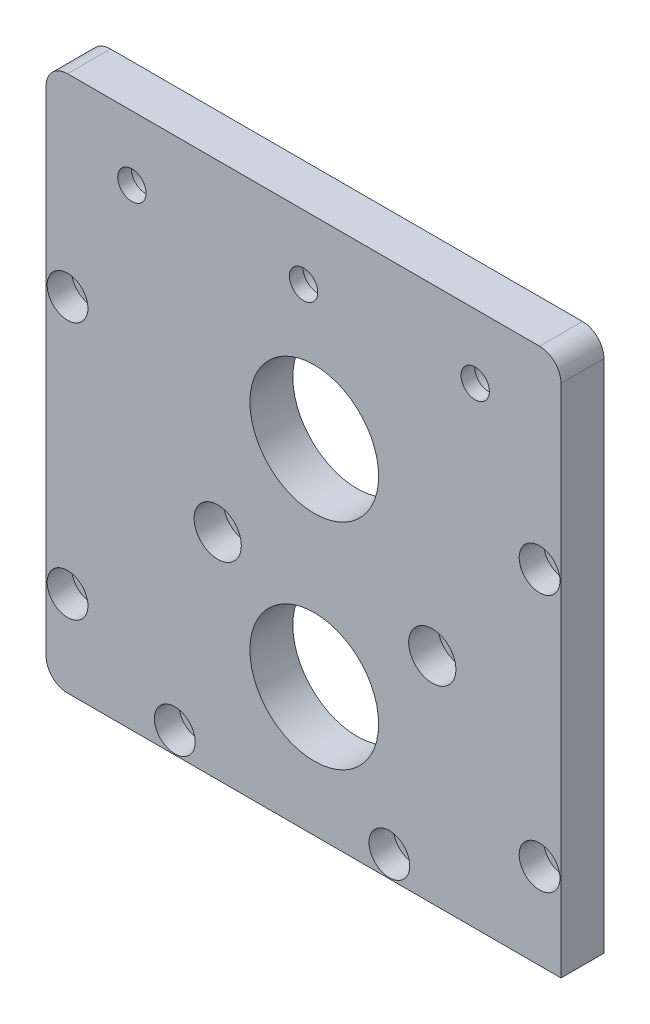
SolidWorks part; units mm, degrees
ref_plane "前视基准面" through (0, 0, 0) normal (0, 0, 1) x (1, 0, 0)
ref_plane "上视基准面" through (0, 0, 0) normal (0, 1, 0) x (1, 0, 0)
ref_plane "右视基准面" through (0, 0, 0) normal (1, 0, 0) x (0, 0, -1)
sketch "草图1" plane through (0, 0, 0) normal (0, 0, 1) x (1, 0, 0)
  line L1 (60, -110) -> (-60, -110)
  line L2 (60, -110) -> (60, 110)
  line L3 (60, 110) -> (-60, 110)
  line L4 (-60, -110) -> (-60, 110)
  line L5 (60, -110) -> (-60, 110) construction
  line L6 (60, 110) -> (-60, -110) construction
  point P0 (0, 0)
  dimension "D1" = 120
  dimension "D2" = 220
extrude "凸台-拉伸1" add sketch "草图1" along normal blind 10
hole_wizard "打孔尺寸(%根据)内六角圆柱头螺钉的类型2" positions "草图7" profile "草图8" counterbore size "M5" standard "GB" end condition up to next
sketch "草图7" plane through (0, 0, 10) normal (0, 0, 1) x (1, 0, 0)
  point P0 (-55, -30)
  point P3 (-55, -90)
sketch "草图8" plane through (-55, -30, 10) normal (1, 0, 0) x (0, -1, 0)
  line L0 (0, 0) -> (0, 10)
  line L1 (0, 10) -> (2.75, 10)
  line L3 (2.75, 10) -> (2.75, 5.7)
  line L4 (2.75, 5.7) -> (4.75, 5.7)
  line L5 (4.75, 5.7) -> (4.75, 0)
  line L7 (4.75, 0) -> (0, 0)
  line L11 (0, -6.35) -> (0, 107.95) construction
  dimension "通孔孔直径" = 5.5
  dimension "通孔孔深度" = 10
  dimension "柱形沉头孔直径" = 9.5
  dimension "柱形沉头孔深度" = 5.7
hole_wizard "打孔尺寸(%根据)内六角圆柱头螺钉的类型3" positions "草图9" profile "草图10" counterbore size "M6" standard "GB" end condition up to next
sketch "草图9" plane through (0, 0, 10) normal (0, 0, 1) x (1, 0, 0)
  point P0 (-20, -60)
  point P3 (30, -60)
sketch "草图10" plane through (-20, -60, 10) normal (1, 0, 0) x (0, -1, 0)
  line L0 (0, 0) -> (0, 10)
  line L1 (0, 10) -> (3.3, 10)
  line L3 (3.3, 10) -> (3.3, 6.8)
  line L4 (3.3, 6.8) -> (5.5, 6.8)
  line L5 (5.5, 6.8) -> (5.5, 0)
  line L7 (5.5, 0) -> (0, 0)
  line L11 (0, -6.35) -> (0, 107.95) construction
  dimension "通孔孔直径" = 6.6
  dimension "通孔孔深度" = 10
  dimension "柱形沉头孔直径" = 11
  dimension "柱形沉头孔深度" = 6.8
fillet "圆角1" radius 5 2 edges at (-60, 110, 5) (-60, -110, 5)
sketch "草图11" plane through (0, 0, 0) normal (0, 0, -1) x (-1, 0, 0)
  line L0 (-60, -110) -> (-60, 110) construction
  line L1 (-60, 15) -> (60, 15)
  line L2 (-60, 15) -> (-60, 110)
  line L3 (-60, 110) -> (60, 110)
  line L4 (60, 15) -> (60, 110)
  line L5 (-60, 110) -> (55, 110) construction
  line L6 (60, 105) -> (60, -105) construction
  dimension "D1" = 95
extrude "切除-拉伸1" cut sketch "草图11" against normal up to next
hole_wizard "打孔尺寸(%根据)内六角圆柱头螺钉的类型4" positions "草图12" profile "草图13" counterbore size "M6" standard "GB" end condition up to next
sketch "草图12" plane through (0, 0, 0) normal (0, 0, -1) x (-1, 0, 0)
  line L0 (-40, 0) -> (0, 0) construction
  line L1 (0, 0) -> (0, 15) construction
  line L2 (-60, 15) -> (60, 15) construction
  line L5 (0, 0) -> (40, 0) construction
  point P0 (-40, 0)
  point P2 (0, 0)
  point P4 (40, 0)
  dimension "D1" = 15
  dimension "D2" = 40
sketch "草图13" plane through (40, 0, 0) normal (1, 0, 0) x (0, 1, 0)
  line L0 (0, 0) -> (0, 10)
  line L1 (0, 10) -> (3.3, 10)
  line L3 (3.3, 10) -> (3.3, 6.8)
  line L4 (3.3, 6.8) -> (5.5, 6.8)
  line L5 (5.5, 6.8) -> (5.5, 0)
  line L7 (5.5, 0) -> (0, 0)
  line L11 (0, -6.35) -> (0, 107.95) construction
  dimension "通孔孔直径" = 6.6
  dimension "通孔孔深度" = 10
  dimension "柱形沉头孔直径" = 11
  dimension "柱形沉头孔深度" = 6.8
fillet "圆角2" radius 5 2 edges at (-60, 15, 5) (60, 15, 5)
sketch "草图14" plane through (0, 0, 0) normal (0, 0, -1) x (-1, 0, 0)
  line L0 (-2.5, -110) -> (-2.5, -80) construction
  line L1 (55, -110) -> (-60, -110) construction
  line L2 (-2.5, -80) -> (-2.5, -30) construction
  circle A0 centre (-2.5, -30) radius 15
  circle A1 centre (-2.5, -80) radius 15
  dimension "D1" = 30
  dimension "D2" = 50
  dimension "D3" = 30
extrude "切除-拉伸2" cut sketch "草图14" against normal up to next
mirror "镜向1" about plane through (0, 0, 0) normal (1, 0, 0) of "打孔尺寸(%根据)内六角圆柱头螺钉的类型2"
hole_wizard "打孔尺寸(%根据)内六角圆柱头螺钉的类型5" positions "草图15" profile "草图16" counterbore size "M5" standard "GB"
sketch "草图15" plane through (0, 0, 10) normal (0, 0, 1) x (1, 0, 0)
  point P0 (20, -105)
  point P3 (-30, -105)
sketch "草图16" plane through (20, -105, 10) normal (1, 0, 0) x (0, -1, 0)
  line L0 (0, 0) -> (0, 22.0524)
  line L1 (0, 22.0524) -> (2.75, 20.4)
  line L2 (2.75, 20.4) -> (2.75, 5.7)
  line L3 (2.75, 5.7) -> (4.75, 5.7)
  line L4 (4.75, 5.7) -> (4.75, 0)
  line L5 (4.75, 0) -> (0, 0)
  line L10 (0, 22.0524) -> (-2.75, 20.4) construction
  line L11 (0, -6.35) -> (0, 107.95) construction
  dimension "孔直径" = 5.5
  dimension "孔深度" = 20.4
  dimension "柱形沉头孔直径" = 9.5
  dimension "柱形沉头孔深度" = 5.7
  dimension "导头角度" = 118
